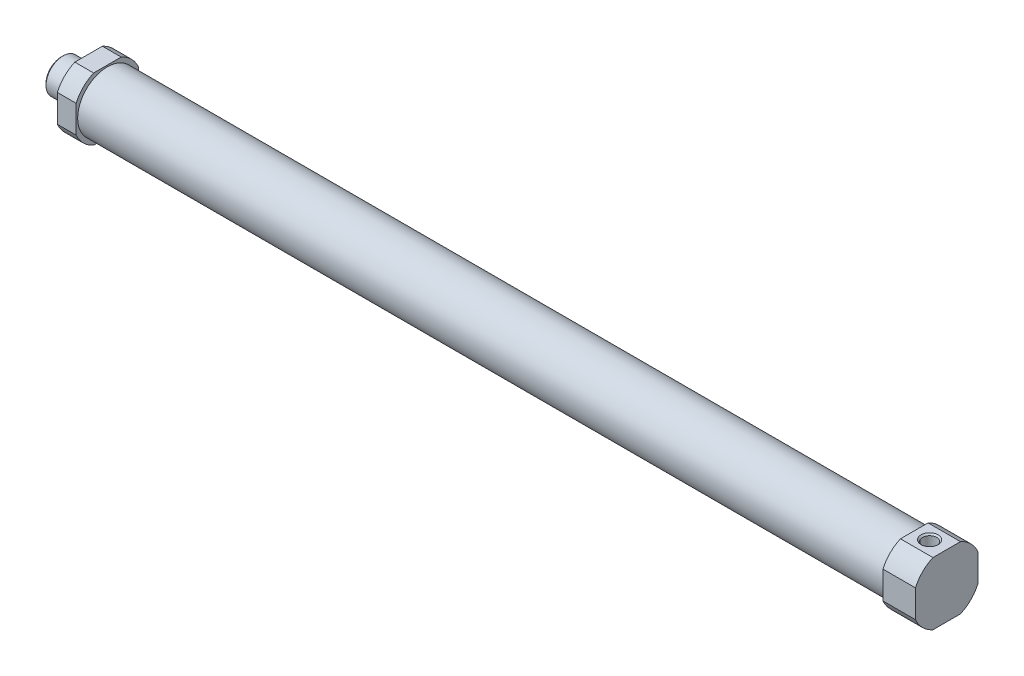
from build123d import *

# Parameters (mm, degrees)
BOSS_EXTRUDE1_DEPTH        = 5.5
SKETCH2_R                  = 8.7
BOSS_EXTRUDE2_DEPTH        = 236
BOSS_EXTRUDE3_DEPTH        = 9.5
SKETCH4_W                  = 8
SKETCH4_H                  = 5
M3_5_CLEARANCE_HOLE1_D     = 4.134
M3_5_CLEARANCE_HOLE1_DEPTH = 5.5
M3_5_CLEARANCE_HOLE1_TIP   = 1.193383006
CHAMFER1_SIZE              = 0.5415
CHAMFER2_SIZE              = 0.433


with BuildPart() as part:
    # Sketch1 → Boss-Extrude1 (new body)
    with BuildSketch(Plane(origin=(0, 0, 0), x_dir=(0, -1, 0), z_dir=(-1, 0, 0))):
        with BuildLine():
            Line((4.034538387, 9.15), (-4.034538387, 9.15))
            ThreePointArc((-4.034538387, 9.15), (-7.071067812, 7.071067812), (-9.15, 4.034538387))
            Line((-9.15, 4.034538387), (-9.15, -4.034538387))
            ThreePointArc((-9.15, -4.034538387), (-7.071067812, -7.071067812), (-4.034538387, -9.15))
            Line((-4.034538387, -9.15), (4.034538387, -9.15))
            ThreePointArc((4.034538387, -9.15), (7.071067812, -7.071067812), (9.15, -4.034538387))
            Line((9.15, -4.034538387), (9.15, 4.034538387))
            ThreePointArc((9.15, 4.034538387), (7.071067812, 7.071067812), (4.034538387, 9.15))
        make_face()
    extrude(amount=-BOSS_EXTRUDE1_DEPTH)

    # Sketch2 → Boss-Extrude2 (add)
    with BuildSketch(Plane(origin=(5.5, 0, 0), x_dir=(0, 0, -1), z_dir=(1, 0, 0))):
        with Locations(Location((0, 0, 0), (0, 0, 180))):
            Circle(SKETCH2_R)
    extrude(amount=BOSS_EXTRUDE2_DEPTH)

    # Sketch3 → Boss-Extrude3 (add)
    with BuildSketch(Plane(origin=(241.5, 0, 0), x_dir=(0, -1, 0), z_dir=(-1, 0, 0))):
        with BuildLine():
            Line((-9.15, 4.034538387), (-9.15, -4.034538387))
            ThreePointArc((-9.15, -4.034538387), (-7.071067812, -7.071067812), (-4.034538387, -9.15))
            Line((-4.034538387, -9.15), (4.034538387, -9.15))
            ThreePointArc((4.034538387, -9.15), (7.071067812, -7.071067812), (9.15, -4.034538387))
            Line((9.15, -4.034538387), (9.15, 4.034538387))
            ThreePointArc((9.15, 4.034538387), (7.071067812, 7.071067812), (4.034538387, 9.15))
            Line((4.034538387, 9.15), (-4.034538387, 9.15))
            ThreePointArc((-4.034538387, 9.15), (-7.071067812, 7.071067812), (-9.15, 4.034538387))
        make_face()
    extrude(amount=-BOSS_EXTRUDE3_DEPTH)

    # Sketch4 → Revolve1 (revolve)
    with BuildSketch(Plane.XY, mode=Mode.PRIVATE) as revolve1_sk:
        with Locations((-4, 2.5)):
            Rectangle(SKETCH4_W, SKETCH4_H)
    revolve(revolve1_sk.sketch.rotate(Axis((-8, 0, 0), (1, 0, 0)), 270), axis=Axis((-8, 0, 0), (1, 0, 0)))

    # M3.5 Clearance Hole1
    with Locations(Plane(origin=(0, 9.15, 0), x_dir=(1, 0, 0), z_dir=(0, 1, 0))):
        with Locations((246, 0)):
            Hole(M3_5_CLEARANCE_HOLE1_D / 2, depth=M3_5_CLEARANCE_HOLE1_DEPTH)
            with Locations((0, 0, -(M3_5_CLEARANCE_HOLE1_DEPTH + M3_5_CLEARANCE_HOLE1_TIP / 2))):  # 120° drill point
                Cone(0, M3_5_CLEARANCE_HOLE1_D / 2, M3_5_CLEARANCE_HOLE1_TIP, mode=Mode.SUBTRACT)

    # Sketch7 → CBORE for M13 SHSS1 (revolve, cut)
    with BuildSketch(Plane(origin=(-8, 0, 0), x_dir=(0, 0, 1), z_dir=(0, 1, 0))):
        Polygon((0, 0), (0, 143.5), (8, 143.5), (8, 13.5), (2.5, 13.5), (2.5, 0), align=None)
    revolve(axis=Axis((-14.35, 0, 0), (1, 0, 0)), mode=Mode.SUBTRACT)

    # Chamfer1
    chamfer1_edges = [part.edges().sort_by_distance(p)[0] for p in [
        (-8, 0, 5),
    ]]
    chamfer(chamfer1_edges, length=CHAMFER1_SIZE)

    # Chamfer2
    chamfer2_edges = [part.edges().sort_by_distance(p)[0] for p in [
        (248.067, 9.15, 0),
    ]]
    chamfer(chamfer2_edges, length=CHAMFER2_SIZE)


solid = part.part
